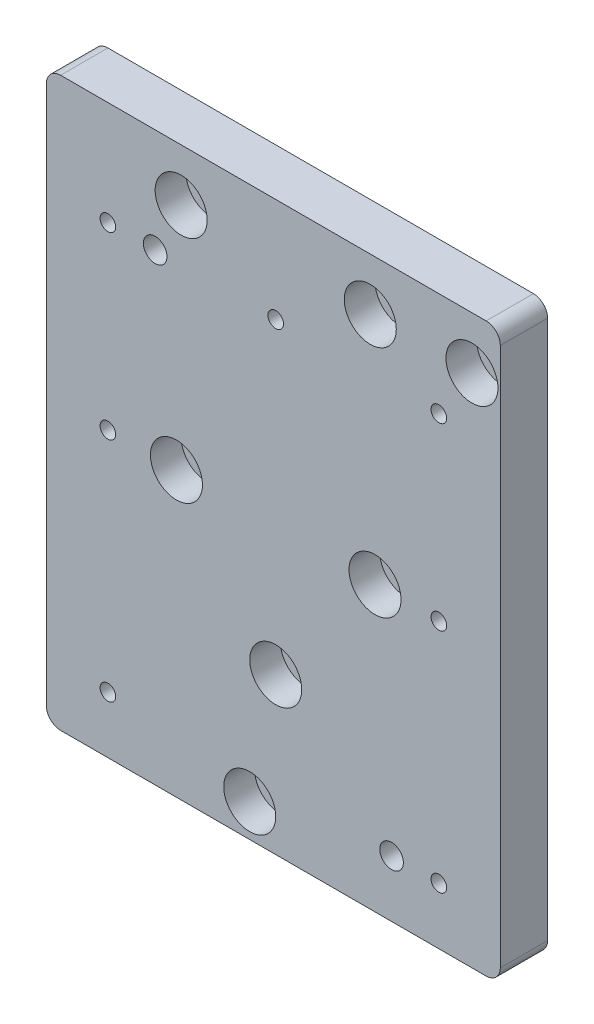
from build123d import *

# Parameters (mm, degrees)
SKETCH_1_W                = 96
SKETCH_1_H                = 120
EXTRUDE_1_DEPTH           = 10
HOLE_WIZARD_2_D           = 6.4
HOLE_WIZARD_2_CBORE_D     = 11
HOLE_WIZARD_2_CBORE_DEPTH = 6.5
FILLET_1_R                = 3
HOLE_WIZARD_M4_1_D        = 3.3
SKETCH_7_R                = 2.5
CUT_EXTRUDE_1_DEPTH       = 10


with BuildPart() as part:
    # 草图1 → 凸台-拉伸1 (new body)
    with BuildSketch(Plane.XY):
        Rectangle(SKETCH_1_W, SKETCH_1_H)
    extrude(amount=EXTRUDE_1_DEPTH)

    # 打孔尺寸(%根据)内六角圆柱头螺钉的类型2 (through all)
    with Locations(Plane.XY.offset(10)):
        with Locations((-19.5, 48.95), (20.5, 48.95), (42, 48.95), (21.5, -0.05), (-20.5, -0.05), (0.5, -27.05), (-5, -53.05)):
            CounterBoreHole(HOLE_WIZARD_2_D / 2, HOLE_WIZARD_2_CBORE_D / 2, HOLE_WIZARD_2_CBORE_DEPTH)

    # 圆角1
    fillet_1_edges = [part.edges().sort_by_distance(p)[0] for p in [
        (48, -60, 5),
        (-48, -60, 5),
        (-48, 60, 5),
        (48, 60, 5),
    ]]
    fillet(fillet_1_edges, radius=FILLET_1_R)

    # M4 螺纹孔1 (through all)
    with Locations(Plane.XY.offset(10)):
        with Locations((-35, -48), (-35, 0), (35, 0), (35, -48), (-35, 38), (35, 38), (0.5, 38)):
            Hole(HOLE_WIZARD_M4_1_D / 2)

    # 草图7 → 切除-拉伸1 (cut)
    with BuildSketch(Plane.XY.offset(10)):
        with Locations((-25, 38)):
            Circle(SKETCH_7_R)
        with Locations((25, -48)):
            Circle(SKETCH_7_R)
    extrude(amount=-CUT_EXTRUDE_1_DEPTH, mode=Mode.SUBTRACT)


solid = part.part
